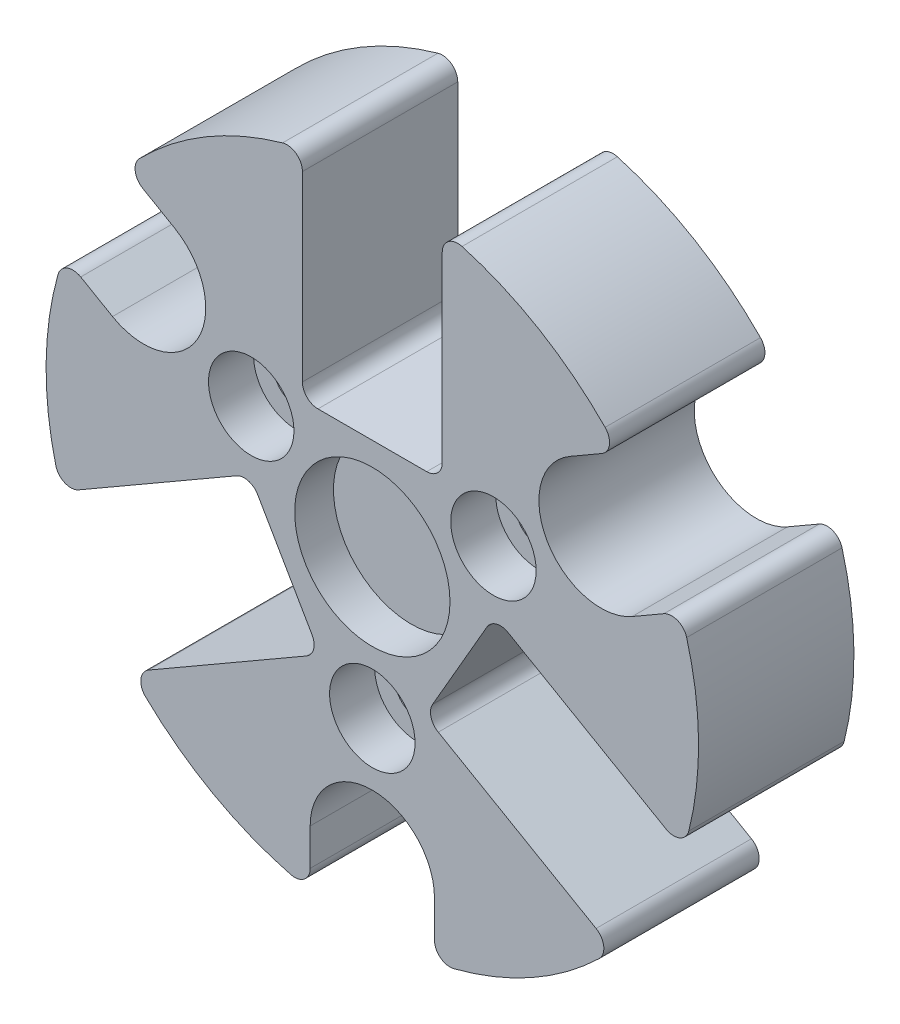
from build123d import *

# Parameters (mm, degrees)
SKETCH1_R                                            = 21
BOSS_EXTRUDE1_DEPTH                                  = 10
SKETCH2_W                                            = 9
SKETCH2_H                                            = 18.909216571
CUT_EXTRUDE1_DEPTH                                   = 12
FILLET1_R                                            = 1
CIRPATTERN1_COUNT                                    = 3
FILLET1_OF_CIRPATTERN1_R                             = 1
CBORE_FOR_M2_5_HEX_SOCKET_HEAD_CAP_SCREW_D           = 2.9
CBORE_FOR_M2_5_HEX_SOCKET_HEAD_CAP_SCREW_CBORE_D     = 5.5
CBORE_FOR_M2_5_HEX_SOCKET_HEAD_CAP_SCREW_CBORE_DEPTH = 2.9
CIRPATTERN2_COUNT                                    = 3
CUT_EXTRUDE2_DEPTH                                   = 32.336879232
FILLET2_R                                            = 1
CIRPATTERN3_COUNT                                    = 3
FILLET2_OF_CIRPATTERN3_R                             = 1
SKETCH7_R                                            = 5
CUT_EXTRUDE4_DEPTH                                   = 2.5


with BuildPart() as part:
    # Sketch1 → Boss-Extrude1 (new body)
    with BuildSketch(Plane.XY):
        Circle(SKETCH1_R)
    extrude(amount=BOSS_EXTRUDE1_DEPTH)

    # Sketch2 → Cut-Extrude1 (cut)
    with BuildSketch(Plane.XY.offset(10)):
        with Locations((0, 15.954608286)):
            Rectangle(SKETCH2_W, SKETCH2_H)
    cut_extrude1 = extrude(amount=-CUT_EXTRUDE1_DEPTH, mode=Mode.SUBTRACT)

    # Fillet1
    fillet1_edges = [part.edges().sort_by_distance(p)[0] for p in [
        (-4.5, 20.512191497, 5),
        (-4.5, 6.5, 5),
        (4.5, 20.512191497, 5),
        (4.5, 6.5, 5),
    ]]
    fillet(fillet1_edges, radius=FILLET1_R)

    # CirPattern1: Cut-Extrude1 ×3 about axis
    cirpattern1_axis = Axis((0, 0, 0), (0, 0, 1))
    for i in range(1, CIRPATTERN1_COUNT):
        add(cut_extrude1.rotate(cirpattern1_axis, i * 360 / CIRPATTERN1_COUNT), mode=Mode.SUBTRACT)

    # Fillet1 of CirPattern1
    fillet1_of_cirpattern1_edges = [part.edges().sort_by_distance(p)[0] for p in [
        (-15.514078923, -14.153210065, 5),
        (-3.379165125, -7.147114317, 5),
        (-20.014078923, -6.358981431, 5),
        (-7.879165125, 0.647114317, 5),
        (20.014078923, -6.358981431, 5),
        (7.879165125, 0.647114317, 5),
        (15.514078923, -14.153210065, 5),
        (3.379165125, -7.147114317, 5),
    ]]
    fillet(fillet1_of_cirpattern1_edges, radius=FILLET1_OF_CIRPATTERN1_R)

    # CBORE for M2.5 Hex Socket Head Cap Screw1 (through all)
    with Locations(Plane.XY.offset(10)):
        with Locations((0, -9)):
            cbore_for_m2_5_hex_socket_head_cap_screw = CounterBoreHole(CBORE_FOR_M2_5_HEX_SOCKET_HEAD_CAP_SCREW_D / 2, CBORE_FOR_M2_5_HEX_SOCKET_HEAD_CAP_SCREW_CBORE_D / 2, CBORE_FOR_M2_5_HEX_SOCKET_HEAD_CAP_SCREW_CBORE_DEPTH)

    # CirPattern2: CBORE for M2.5 Hex Socket Head Cap Screw1 ×3 about axis
    cirpattern2_axis = Axis((0, 0, 0), (0, 0, 1))
    for i in range(1, CIRPATTERN2_COUNT):
        add(cbore_for_m2_5_hex_socket_head_cap_screw.rotate(cirpattern2_axis, i * 360 / CIRPATTERN2_COUNT), mode=Mode.SUBTRACT)

    # Sketch5 → Cut-Extrude2 (cut, through all)
    with BuildSketch(Plane.XY.offset(10)):
        with BuildLine():
            Line((4, -17), (4, -24.000575883))
            ThreePointArc((4, -24.000575883), (0, -28.000575883), (-4, -24.000575883))
            Line((-4, -24.000575883), (-4, -17))
            ThreePointArc((-4, -17), (0, -13), (4, -17))
        make_face()
    cut_extrude2 = extrude(amount=-CUT_EXTRUDE2_DEPTH, mode=Mode.SUBTRACT)

    # Fillet2
    fillet2_edges = [part.edges().sort_by_distance(p)[0] for p in [
        (4, -20.615528128, 5),
        (-4, -20.615528128, 5),
    ]]
    fillet(fillet2_edges, radius=FILLET2_R)

    # CirPattern3: Cut-Extrude2 ×3 about axis
    cirpattern3_axis = Axis((0, 0, 0), (0, 0, 1))
    for i in range(1, CIRPATTERN3_COUNT):
        add(cut_extrude2.rotate(cirpattern3_axis, i * 360 / CIRPATTERN3_COUNT), mode=Mode.SUBTRACT)

    # Fillet2 of CirPattern3
    fillet2_of_cirpattern3_edges = [part.edges().sort_by_distance(p)[0] for p in [
        (15.853571071, 13.771865679, 5),
        (19.853571071, 6.843662449, 5),
        (-19.853571071, 6.843662449, 5),
        (-15.853571071, 13.771865679, 5),
    ]]
    fillet(fillet2_of_cirpattern3_edges, radius=FILLET2_OF_CIRPATTERN3_R)

    # Sketch7 → Cut-Extrude4 (cut)
    with BuildSketch(Plane.XY.offset(10)):
        Circle(SKETCH7_R)
    extrude(amount=-CUT_EXTRUDE4_DEPTH, mode=Mode.SUBTRACT)


solid = part.part
